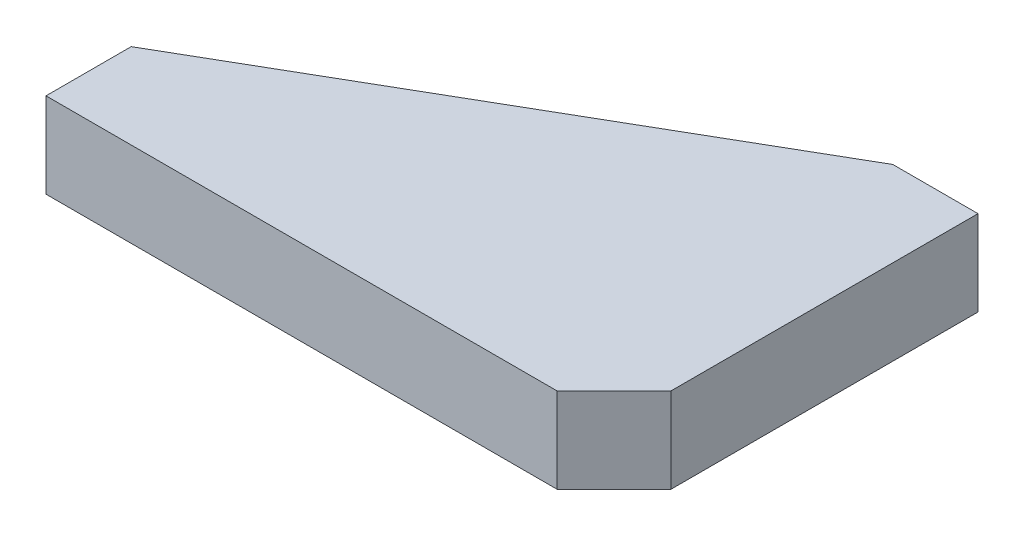
from build123d import *

# Parameters (mm, degrees)
EXTRUDE_1_DEPTH = 30


with BuildPart() as part:
    # 草图1 → 凸台-拉伸1 (new body)
    with BuildSketch(Plane(origin=(0, 0, 0), x_dir=(1, 0, 0), z_dir=(0, 1, 0))):
        Polygon((0, 0), (-30, 0), (-200, -98.149545762), (-200, -128.149545762), (-20, -128.149545762), (0, -108.149545762), align=None)
    extrude(amount=EXTRUDE_1_DEPTH)


solid = part.part
